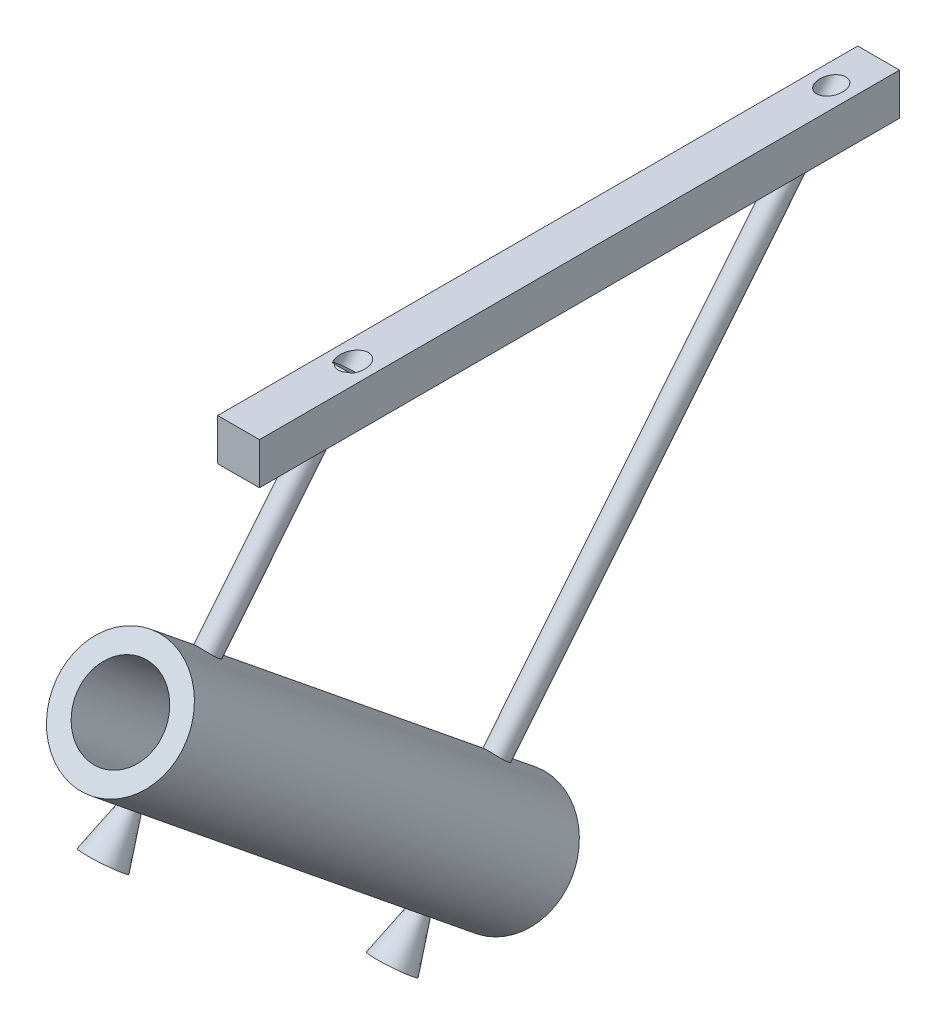
SolidWorks part; units mm, degrees
ref_plane "Front Plane" through (0, 0, 0) normal (0, 0, 1) x (1, 0, 0)
ref_plane "Top Plane" through (0, 0, 0) normal (0, 1, 0) x (1, 0, 0)
ref_plane "Right Plane" through (0, 0, 0) normal (1, 0, 0) x (0, 0, -1)
sketch "Sketch2" plane through (0, 0, 0) normal (0, 1, 0) x (1, 0, 0)
  line L1 (0, 0) -> (-15, 0)
  line L2 (0, 0) -> (0, -230)
  line L3 (0, -230) -> (-15, -230)
  line L4 (-15, 0) -> (-15, -230)
  dimension "D1" = 15
  dimension "D2" = 230
extrude "Boss-Extrude2" add sketch "Sketch2" along normal blind 15
sketch "Sketch3" plane through (0, 15, 0) normal (0, 1, 0) x (1, 0, 0)
  line L0 (-7.5, 0) -> (-7.5, -230)
  line L1 (0, 0) -> (-15, 0) construction
  line L2 (-15, -230) -> (0, -230) construction
ref_plane "Plane1" through (0, -112.487, 91.0902) normal (0, 0.7771, -0.6293) x (1, 0, 0)
sketch "Sketch4" plane through (0, -112.487, 91.0902) normal (0, 0.7771, -0.6293) x (1, 0, 0)
  line L0 (-7.5, -9.4398) -> (-7.5, -188.1834) construction
  circle A3 centre (-7.5, -22.6654) radius 4
  circle A4 centre (-7.5, -156.3759) radius 4
extrude "Boss-Extrude3" add sketch "Sketch4" along normal mid plane 310
sketch "Sketch5" plane through (0, 7.9706, -6.4545) normal (0, 0.7771, -0.6293) x (1, 0, 0)
  circle A0 centre (-7.5, -156.3759) radius 4.4738
extrude "Cut-Extrude1" cut sketch "Sketch5" against normal blind 120
sketch "Sketch6" plane through (0, 7.9706, -6.4545) normal (0, 0.7771, -0.6293) x (1, 0, 0)
  circle A0 centre (-7.5, -22.6654) radius 4.1
extrude "Cut-Extrude2" cut sketch "Sketch6" against normal blind 17
sketch "Sketch7" plane through (0, -232.9446, 188.6348) normal (0, -0.7771, 0.6293) x (1, 0, 0)
  circle A0 centre (-7.5, 22.6654) radius 5.3114
  circle A1 centre (-7.5, 156.3759) radius 5.67
extrude "Cut-Extrude3" cut sketch "Sketch7" against normal blind 62
ref_plane "Plane2" through (0, 112.487, 138.9098) normal (0, -0.6293, -0.7771) x (1, 0, 0)
sketch "Sketch8" plane through (0, 112.487, 138.9098) normal (0, -0.6293, -0.7771) x (1, 0, 0)
  circle A3 centre (-7.5, 212.1985) radius 22.5
extrude "Boss-Extrude4" add sketch "Sketch8" along normal blind 178
sketch "Sketch9" plane through (0, -184.7615, 149.617) normal (0, -0.7771, 0.6293) x (1, 0, 0)
  circle A0 centre (-7.5, 156.3759) radius 4.2
  circle A1 centre (-7.5, 22.6654) radius 4.2
extrude "Cut-Extrude4" cut sketch "Sketch9" against normal blind 8
sketch "Sketch10" plane through (0, -178.5444, 144.5824) normal (0, -0.7771, 0.6293) x (1, 0, 0)
  circle A0 centre (-7.5, 156.3759) radius 2
  circle A1 centre (-7.5, 22.6654) radius 2
extrude "Boss-Extrude5" add sketch "Sketch10" along normal blind 20 draft 15 draft outward yes
sketch "Sketch11" plane through (0, 112.487, 138.9098) normal (0, 0.6293, 0.7771) x (1, 0, 0)
  circle A0 centre (-7.5, -212.1985) radius 15
extrude "Cut-Extrude5" cut sketch "Sketch11" against normal blind 193
sketch "Sketch12" plane through (0, 112.487, 138.9098) normal (0, 0.6293, 0.7771) x (1, 0, 0)
  line L0 (-7.5, -189.6985) -> (-7.5, -234.6985)
  arc A0 (-3.5, -190.057) -> (-11.5, -190.057) centre (-7.5, -212.1985) ccw construction
  circle A1 centre (-7.5, -212.1985) radius 22.5 construction
